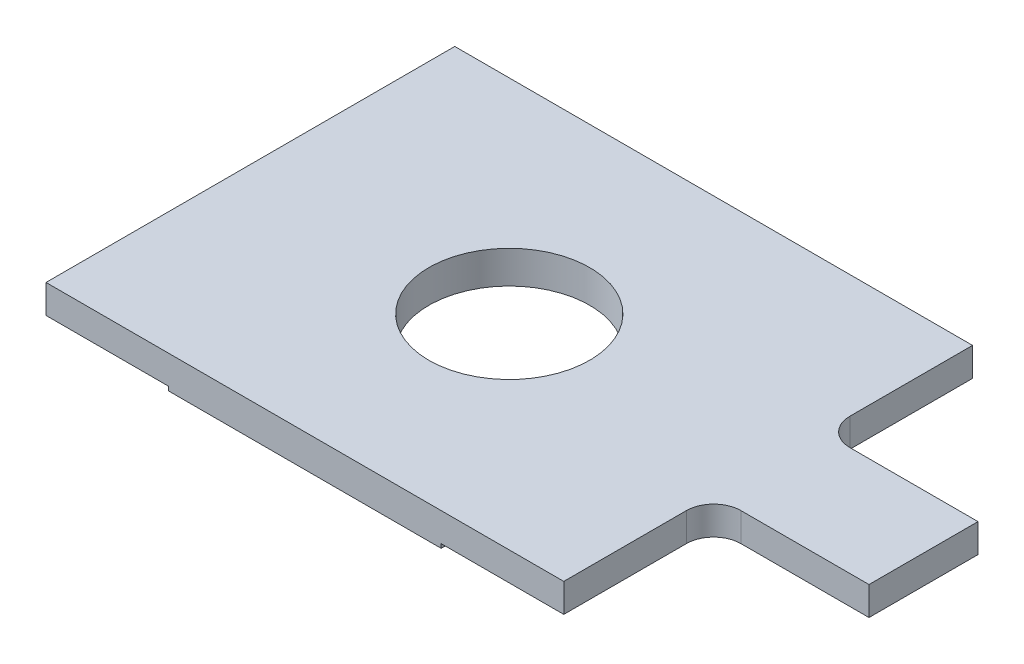
SolidWorks part; units mm, degrees
ref_plane "前视基准面" through (0, 0, 0) normal (0, 0, 1) x (1, 0, 0)
ref_plane "上视基准面" through (0, 0, 0) normal (0, 1, 0) x (1, 0, 0)
ref_plane "右视基准面" through (0, 0, 0) normal (1, 0, 0) x (0, 0, -1)
sketch "草图1" plane through (0, 0, 0) normal (0, 0, 1) x (1, 0, 0)
  line L0 (0, 0) -> (-50, 0)
  line L1 (-50, 0) -> (-50, 1.5)
  line L2 (-50, 1.5) -> (-95, 1.5)
  line L3 (-95, 1.5) -> (-95, 12)
  line L4 (-95, 12) -> (95, 12)
  line L5 (95, 12) -> (95, 1.5)
  line L6 (95, 1.5) -> (50, 1.5)
  line L7 (50, 1.5) -> (50, 0)
  line L8 (50, 0) -> (0, 0)
  dimension "D1" = 100
  dimension "D2" = 190
  dimension "D3" = 1.5
  dimension "D4" = 12
extrude "凸台-拉伸1" add sketch "草图1" along normal mid plane 150
sketch "草图2" plane through (0, 12, 0) normal (0, 1, 0) x (1, 0, 0)
  circle A0 centre (0, 0) radius 29.5
  dimension "D1" = 59
extrude "切除-拉伸1" cut sketch "草图2" against normal up to next
sketch "草图4" plane through (95, 0, 0) normal (1, 0, 0) x (0, 0, -1)
  line L0 (-75, 12) -> (75, 12) construction
  line L1 (-20, 12) -> (20, 12)
  line L2 (-20, 12) -> (-20, 1.5)
  line L3 (-20, 1.5) -> (20, 1.5)
  line L4 (20, 12) -> (20, 1.5)
  line L6 (-75, 1.5) -> (75, 1.5) construction
  line L7 (0, 12) -> (0, 0) construction
  dimension "D1" = 40
extrude "凸台-拉伸2" add sketch "草图4" along normal blind 57
fillet "圆角1" radius 10 2 edges at (95, 6.75, -20) (95, 6.75, 20)
